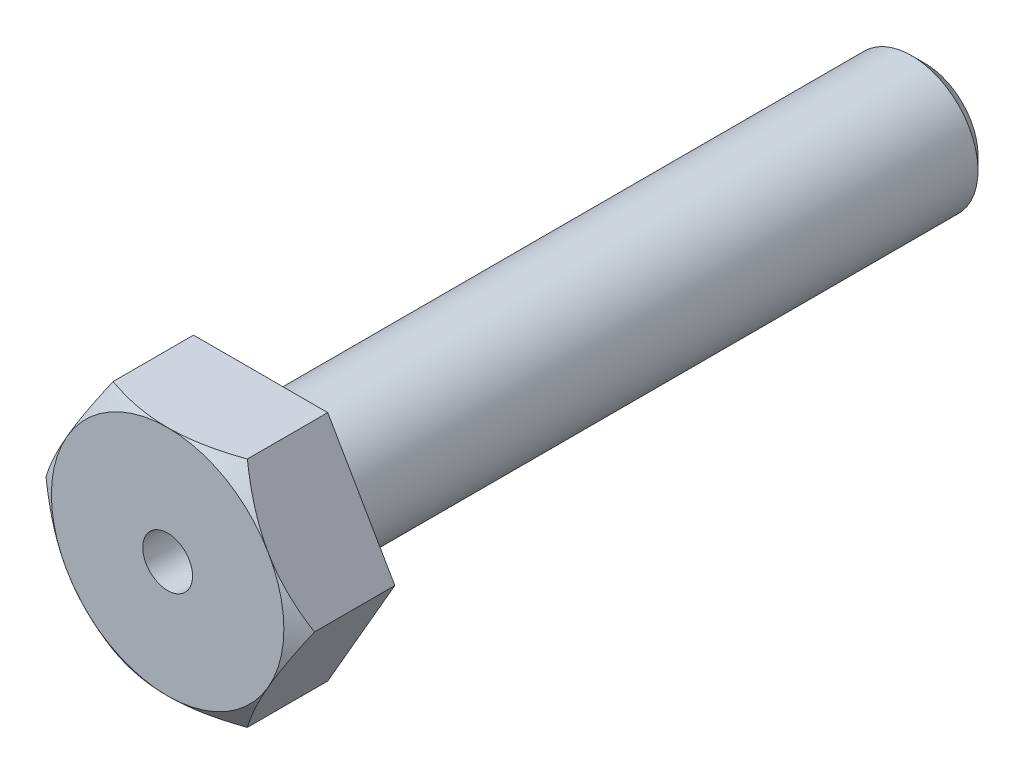
SolidWorks part; units mm, degrees
ref_plane "Front Plane" through (0, 0, 0) normal (0, 0, 1) x (1, 0, 0)
ref_plane "Top Plane" through (0, 0, 0) normal (0, 1, 0) x (1, 0, 0)
ref_plane "Right Plane" through (0, 0, 0) normal (1, 0, 0) x (0, 0, -1)
sketch "Sketch1" plane through (0, 0, 0) normal (1, 0, 0) x (0, 0, -1)
  line L0 (-2.8, 0) -> (20, 0) construction
  line L1 (-2.8, 0) -> (-2.8, 3.5)
  line L2 (-2.8, 3.5) -> (0, 3.5)
  line L3 (0, 3.5) -> (0, 2)
  line L4 (0, 2) -> (20, 2)
  line L5 (20, 2) -> (20, 0)
  point P10 (20, 0.75)
  dimension "A" = 7
  dimension "E" = 2.8
  dimension "L" = 20
  dimension "M" = 4
  dimension "(d)" = 1.5
sketch "Sketch3" plane through (0, 0, 0) normal (1, 0, 0) x (0, 0, -1)
  line L2 (0, 2) -> (20, 2) construction
  line L4 (0, 2) -> (-2.8, 2)
  line L5 (20, 2) -> (20, 0) construction
  line L6 (-2.8, 2) -> (-2.8, 0.75)
  line L8 (0, 2) -> (20, 2)
  line L10 (20, 0.75) -> (-2.8, 0.75)
  line L11 (20, 2) -> (20, 0.75)
revolve "Revolve1" add sketch "Sketch3" angle 360 about L0
cosmetic thread "Cosmetic Thread1" parameters "D1"=20, "D2"=3.4
sketch "Sketch4" plane through (0, 0, 2.8) normal (0, 0, 1) x (1, 0, 0)
  line L7 (2.0207, 3.5) -> (-2.0207, 3.5)
  line L8 (-2.0207, 3.5) -> (-4.0415, 0)
  line L9 (-4.0415, 0) -> (-2.0207, -3.5)
  line L10 (-2.0207, -3.5) -> (2.0207, -3.5)
  line L11 (2.0207, -3.5) -> (4.0415, 0)
  line L12 (4.0415, 0) -> (2.0207, 3.5)
  circle A0 centre (0, 0) radius 3.5 construction
  circle A1 centre (0, 0) radius 0.75
extrude "Boss-Extrude1" add sketch "Sketch4" against normal up to vertex (2.8 mm away) up to point (0, 3.5, 0)
sketch "Sketch5" plane through (0, 0, 2.8) normal (0, 0, 1) x (1, 0, 0)
  line L0 (-3.5, 0) -> (-4.0415, 0) construction
  line L1 (-4.0415, 0) -> (-4.5829, 0) construction
  circle A0 centre (0, 0) radius 3.5
  circle A1 centre (0, 0) radius 4.5829
  circle A2 centre (0, 0) radius 3.5 construction
extrude "Cut-Extrude1" cut sketch "Sketch5" against normal blind 1 draft 55
chamfer "Chamfer1" distance 0.4 angle 45 1 edges at (0, -2, -20)
